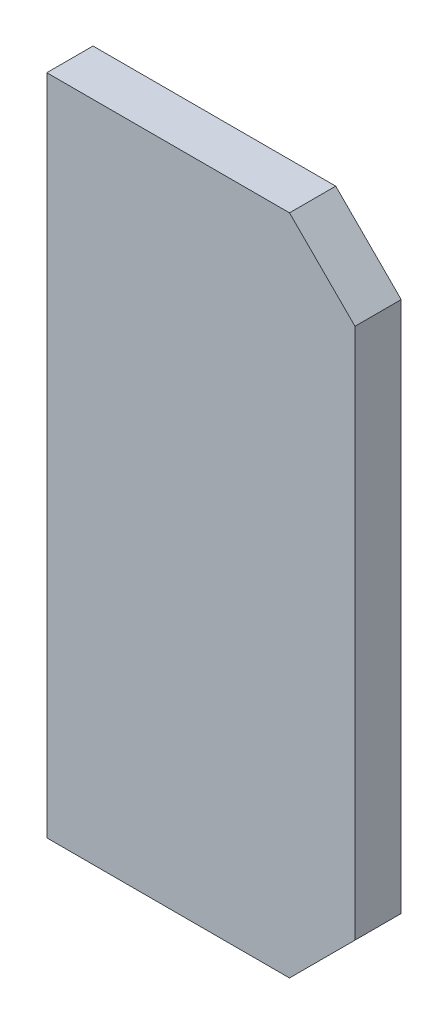
from build123d import *

# Parameters (mm, degrees)
SKETCH1_W           = 40
SKETCH1_H           = 86
BOSS_EXTRUDE1_DEPTH = 6
CHAMFER1_SIZE       = 8.5


with BuildPart() as part:
    # Sketch1 → Boss-Extrude1 (new body)
    with BuildSketch(Plane.XY):
        Rectangle(SKETCH1_W, SKETCH1_H)
    extrude(amount=BOSS_EXTRUDE1_DEPTH)

    # Chamfer1
    chamfer1_edges = [part.edges().sort_by_distance(p)[0] for p in [
        (20, 43, 3),
        (20, -43, 3),
    ]]
    chamfer(chamfer1_edges, length=CHAMFER1_SIZE)


solid = part.part
